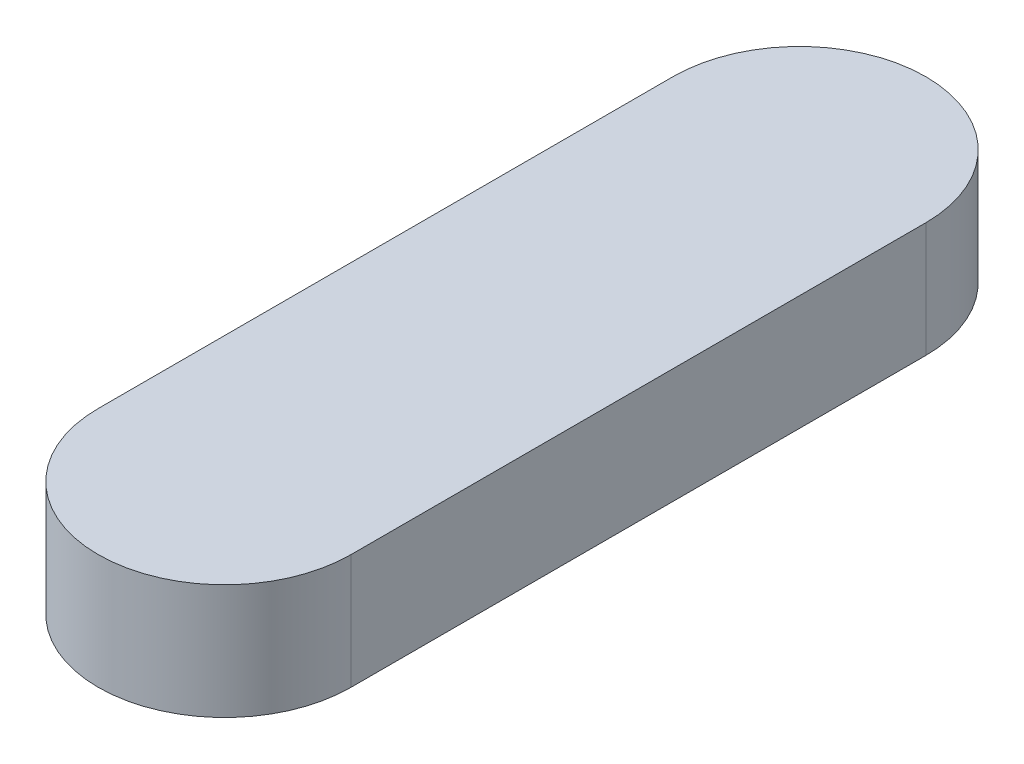
from build123d import *

# Parameters (mm, degrees)
BOSS_EXTRUDE1_DEPTH = 10


with BuildPart() as part:
    # Sketch1 → Boss-Extrude1 (new body)
    with BuildSketch(Plane(origin=(0, 0, 0), x_dir=(1, 0, 0), z_dir=(0, 1, 0))):
        with BuildLine():
            Line((-11, -25), (-11, 25))
            ThreePointArc((-11, 25), (0, 36), (11, 25))
            Line((11, 25), (11, -25))
            ThreePointArc((11, -25), (0, -36), (-11, -25))
        make_face()
    extrude(amount=BOSS_EXTRUDE1_DEPTH)


solid = part.part
